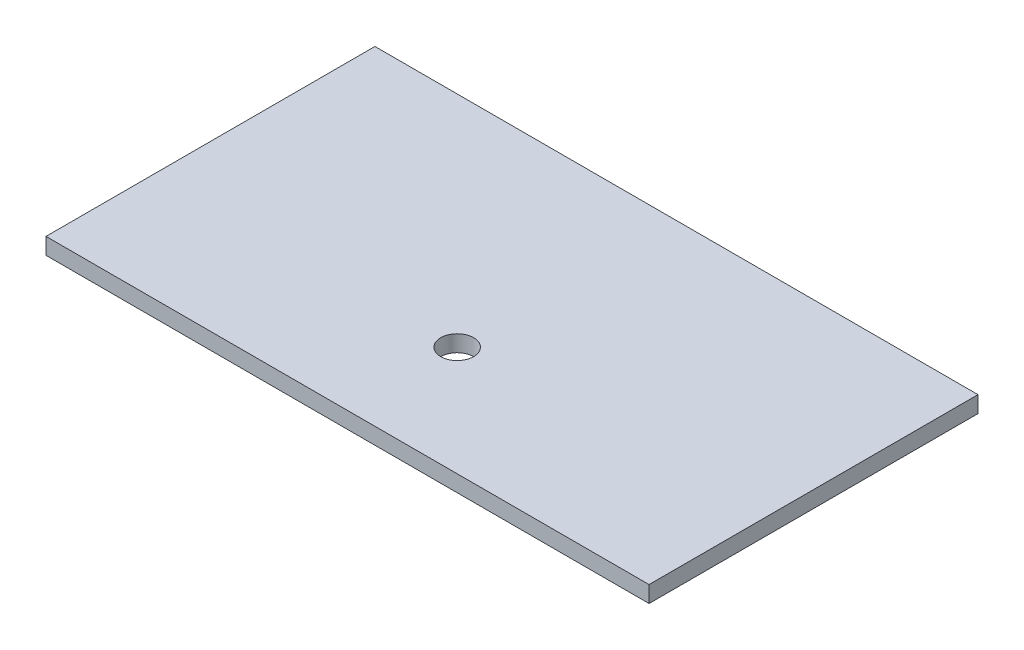
from build123d import *

# Parameters (mm, degrees)
SKETCH1_W           = 110
SKETCH1_H           = 60
SKETCH1_R           = 3
BOSS_EXTRUDE1_DEPTH = 3


with BuildPart() as part:
    # Sketch1 → Boss-Extrude1 (new body)
    with BuildSketch(Plane(origin=(0, 0, 0), x_dir=(1, 0, 0), z_dir=(0, 1, 0))):
        Rectangle(SKETCH1_W, SKETCH1_H)
        with Locations(Location((0, -10, 0), (0, 0, 270))):
            Circle(SKETCH1_R, mode=Mode.SUBTRACT)
    extrude(amount=BOSS_EXTRUDE1_DEPTH)


solid = part.part
